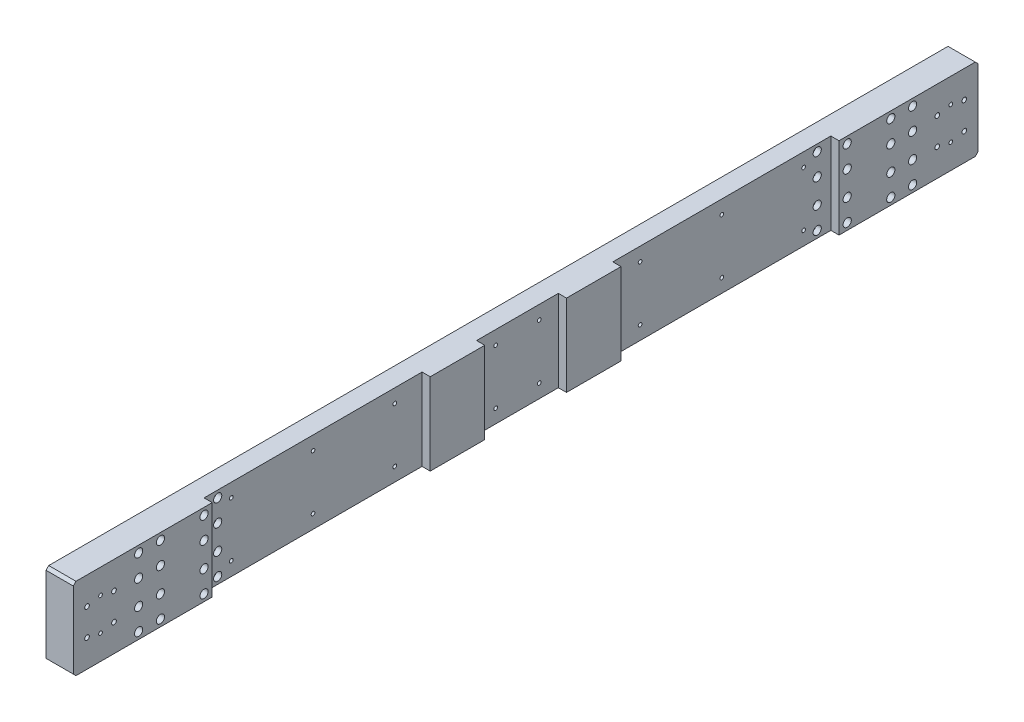
from build123d import *

# Parameters (mm, degrees)
SKETCH_1_W                  = 1660
SKETCH_1_H                  = 150
EXTRUDE_1_DEPTH             = 50
HOLE_WIZARD_M10_1_D         = 8.5
SKETCH_4_W                  = 150
SKETCH_4_H                  = 150
SKETCH_4_W_2                = 400
CUT_EXTRUDE_1_DEPTH         = 15
HOLE_WIZARD_M8_1_D          = 6.8
HOLE_WIZARD_M8_2_D          = 6.8
HOLE_WIZARD_1_D             = 9
HOLE_WIZARD_1_CBORE_D       = 15
HOLE_WIZARD_1_CBORE_DEPTH   = 25
PATTERN_LINEAR_1_COUNT      = 2
PATTERN_LINEAR_1_PITCH      = 120
MIRROR_3_COPY_1_D           = 9
MIRROR_3_COPY_1_CBORE_D     = 15
MIRROR_3_COPY_1_CBORE_DEPTH = 25
HOLE_WIZARD_M8_3_D          = 6.8
CHAMFER_1_SIZE              = 5


with BuildPart() as part:
    # 草图1 → 凸台-拉伸1 (new body)
    with BuildSketch(Plane(origin=(0, 0, 0), x_dir=(0, 0, -1), z_dir=(1, 0, 0))):
        Rectangle(SKETCH_1_W, SKETCH_1_H)
    extrude(amount=EXTRUDE_1_DEPTH)

    # M10 螺纹孔1 (through all)
    with Locations(Plane(origin=(50, 0, 0), x_dir=(0, 0, -1), z_dir=(1, 0, 0))):
        with Locations((-804.748737342, 24.748737342), (-755.251262658, 24.748737342), (-804.748737342, -24.748737342), (-755.251262658, -24.748737342)):
            hole_wizard_m10_1 = Hole(HOLE_WIZARD_M10_1_D / 2)

    # 镜向1: M10 螺纹孔1 across plane
    add(hole_wizard_m10_1.mirror(Plane.XY), mode=Mode.SUBTRACT)

    # 草图4 → 切除-拉伸1 (cut)
    with BuildSketch(Plane(origin=(50, 0, 0), x_dir=(0, 0, -1), z_dir=(1, 0, 0))):
        Rectangle(SKETCH_4_W, SKETCH_4_H)
        with Locations((-375, 0)):
            Rectangle(SKETCH_4_W_2, SKETCH_4_H)
        with Locations((375, 0)):
            Rectangle(SKETCH_4_W_2, SKETCH_4_H)
    extrude(amount=-CUT_EXTRUDE_1_DEPTH, mode=Mode.SUBTRACT)

    # M8 螺纹孔1 (through all)
    with Locations(Plane(origin=(35, 0, 0), x_dir=(0, 0, -1), z_dir=(1, 0, 0))):
        with Locations((-525, 50), (-375, 50), (-225, 50), (-525, -50), (-375, -50), (-225, -50)):
            hole_wizard_m8_1 = Hole(HOLE_WIZARD_M8_1_D / 2)

    # 镜向2: M8 螺纹孔1 across plane
    add(hole_wizard_m8_1.mirror(Plane.XY), mode=Mode.SUBTRACT)

    # M8 螺纹孔2 (through all)
    with Locations(Plane(origin=(35, 0, 0), x_dir=(0, 0, -1), z_dir=(1, 0, 0))):
        with Locations((-40, 50), (40, 50), (-40, -50), (40, -50)):
            Hole(HOLE_WIZARD_M8_2_D / 2)

    # 打孔尺寸(%根据)内六角圆柱头螺钉的类型1 (through all)
    with Locations(Plane(origin=(50, 0, 0), x_dir=(0, 0, -1), z_dir=(1, 0, 0))):
        with Locations((-710, -22.5), (-710, -62.5), (-670, -22.5), (-670, -62.5), (-670, 62.5), (-670, 22.5), (-710, 62.5), (-710, 22.5)):
            hole_wizard_1 = CounterBoreHole(HOLE_WIZARD_1_D / 2, HOLE_WIZARD_1_CBORE_D / 2, HOLE_WIZARD_1_CBORE_DEPTH)

    # 阵列(线性)1: 打孔尺寸(%根据)内六角圆柱头螺钉的类型1 ×2
    with Locations(*[(0, 0, -i * PATTERN_LINEAR_1_PITCH) for i in range(1, PATTERN_LINEAR_1_COUNT)]):
        add(hole_wizard_1, mode=Mode.SUBTRACT)

    # 镜向3: 打孔尺寸(%根据)内六角圆柱头螺钉的类型1 across plane
    add(hole_wizard_1.mirror(Plane.XY), mode=Mode.SUBTRACT)

    # 镜向3 copy 1 (through all)
    with Locations(Plane(origin=(50, 0, 120), x_dir=(0, 0, 1), z_dir=(1, 0, 0))):
        with Locations((-710, 22.5), (-710, 62.5), (-670, 22.5), (-670, 62.5), (-670, -62.5), (-670, -22.5), (-710, -62.5), (-710, -22.5)):
            CounterBoreHole(MIRROR_3_COPY_1_D / 2, MIRROR_3_COPY_1_CBORE_D / 2, MIRROR_3_COPY_1_CBORE_DEPTH)

    # M8 螺纹孔3 (through all)
    with Locations(Plane(origin=(50, 0, 0), x_dir=(0, 0, -1), z_dir=(1, 0, 0))):
        with Locations((-780, 30), (-780, -30)):
            hole_wizard_m8_3 = Hole(HOLE_WIZARD_M8_3_D / 2)

    # 镜向4: M8 螺纹孔3 across plane
    add(hole_wizard_m8_3.mirror(Plane.XY), mode=Mode.SUBTRACT)

    # 倒角1
    chamfer_1_edges = [part.edges().sort_by_distance(p)[0] for p in [
        (25, -75, -830),
        (25, -75, 830),
        (25, 75, 830),
        (25, 75, -830),
    ]]
    chamfer(chamfer_1_edges, length=CHAMFER_1_SIZE)


solid = part.part
